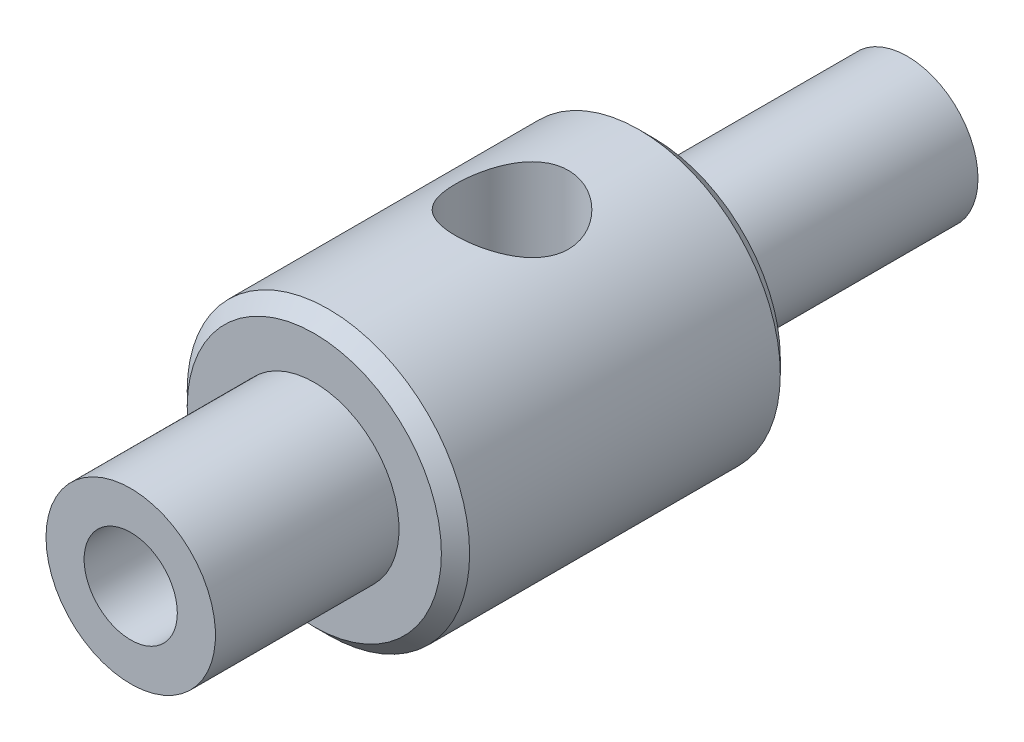
SolidWorks part; units mm, degrees
material "S45C"
ref_plane "Front Plane" through (0, 0, 0) normal (0, 0, 1) x (1, 0, 0)
ref_plane "Top Plane" through (0, 0, 0) normal (0, 1, 0) x (1, 0, 0)
ref_plane "Right Plane" through (0, 0, 0) normal (1, 0, 0) x (0, 0, -1)
sketch "Sketch1" plane through (0, 0, 0) normal (0, 0, 1) x (1, 0, 0)
  circle A0 centre (0, 0) radius 5
  dimension "D1" = 10
extrude "Boss-Extrude1" add sketch "Sketch1" along normal blind 12
sketch "Sketch2" plane through (0, 0, 12) normal (0, 0, 1) x (1, 0, 0)
  circle A0 centre (0, 0) radius 3
  dimension "D1" = 6
extrude "Boss-Extrude2" add sketch "Sketch2" along normal blind 6.5
hole_wizard "M4 Tapped Hole1" positions "Sketch4" profile "Sketch3" tap size "M4" standard "GB"
sketch "Sketch4" plane through (0, 0, 18.5) normal (0, 0, 1) x (1, 0, 0)
  point P0 (0, 0)
sketch "Sketch3" plane through (0, 0, 18.5) normal (1, 0, 0) x (0, -1, 0)
  line L0 (0, 0) -> (0, 11.0914)
  line L1 (0, 11.0914) -> (1.65, 10.1)
  line L2 (1.65, 10.1) -> (1.65, 0)
  line L5 (1.65, 0) -> (0, 0)
  line L10 (0, 11.0914) -> (-1.65, 10.1) construction
  line L11 (0, -6.35) -> (0, 107.95) construction
  dimension "螺纹孔钻头直径" = 3.3
  dimension "螺纹孔钻头深度" = 10.1
  dimension "导头角度" = 118
cosmetic thread "孔螺蚊线1" parameters "D1"=8, "D2"=4
sketch "Sketch5" plane through (0, 0, 0) normal (0, 0, -1) x (-1, 0, 0)
  circle A0 centre (0, 0) radius 2.5
  dimension "D1" = 5
extrude "Boss-Extrude3" add sketch "Sketch5" along normal blind 9
cosmetic thread "Cosmetic Thread1" parameters "D1"=8, "D2"=4.134
sketch "Sketch6" plane through (0, 0, 0) normal (0, 1, 0) x (1, 0, 0)
  line L0 (5, 0) -> (-5, 0) construction
  circle A0 centre (0, -5) radius 2
  dimension "D1" = 4
  dimension "D2" = 5
extrude "Cut-Extrude1" cut sketch "Sketch6" against normal mid plane 15
chamfer "Chamfer1" distance 0.5 angle 45 2 edges at (5, 0, 12) (5, 0, 0)
